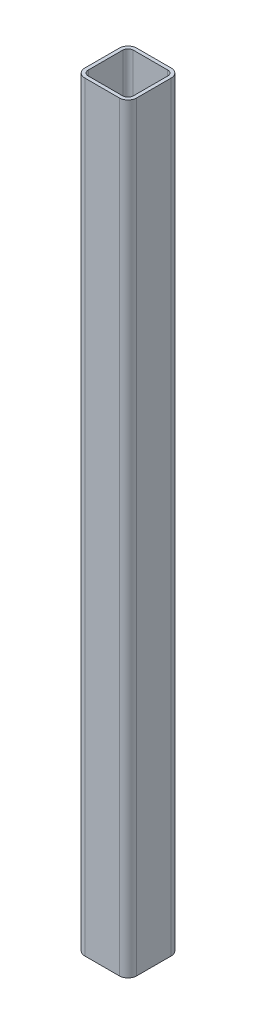
from build123d import *

# Parameters (mm, degrees)
BOSS_EXTRUDE1_DEPTH = 880


with BuildPart() as part:
    # Sketch1 → Boss-Extrude1 (new body)
    with BuildSketch(Plane(origin=(0, 0, 0), x_dir=(1, 0, 0), z_dir=(0, 1, 0))):
        with BuildLine():
            Line((-20, -30), (20, -30))
            ThreePointArc((20, -30), (27.071067812, -27.071067812), (30, -20))
            Line((30, -20), (30, 20))
            ThreePointArc((30, 20), (27.071067812, 27.071067812), (20, 30))
            Line((20, 30), (-20, 30))
            ThreePointArc((-20, 30), (-27.071067812, 27.071067812), (-30, 20))
            Line((-30, 20), (-30, -20))
            ThreePointArc((-30, -20), (-27.071067812, -27.071067812), (-20, -30))
        make_face()
        with BuildLine():
            Line((-26, -20), (-26, 20))
            ThreePointArc((-26, 20), (-24.242640687, 24.242640687), (-20, 26))
            Line((-20, 26), (20, 26))
            ThreePointArc((20, 26), (24.242640687, 24.242640687), (26, 20))
            Line((26, 20), (26, -20))
            ThreePointArc((26, -20), (24.242640687, -24.242640687), (20, -26))
            Line((20, -26), (-20, -26))
            ThreePointArc((-20, -26), (-24.242640687, -24.242640687), (-26, -20))
        make_face(mode=Mode.SUBTRACT)
    extrude(amount=BOSS_EXTRUDE1_DEPTH)


solid = part.part
